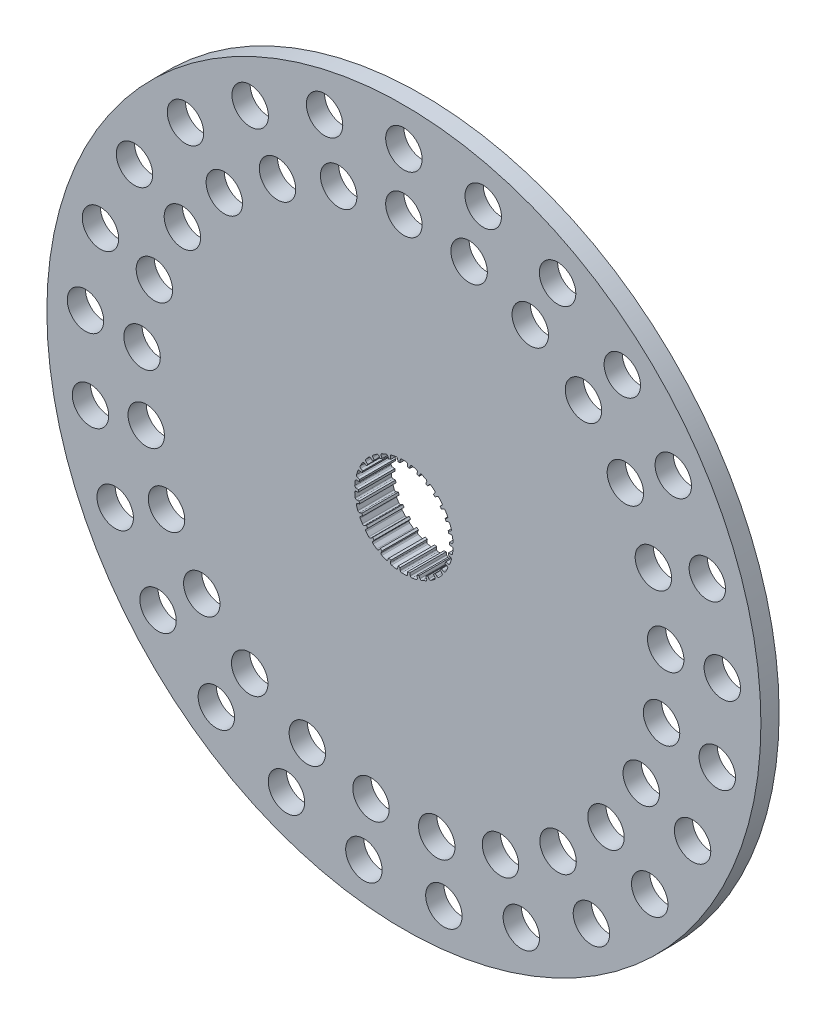
SolidWorks part; units mm, degrees
ref_plane "Front Plane" through (0, 0, 0) normal (0, 0, 1) x (1, 0, 0)
ref_plane "Top Plane" through (0, 0, 0) normal (0, 1, 0) x (1, 0, 0)
ref_plane "Right Plane" through (0, 0, 0) normal (1, 0, 0) x (0, 0, -1)
sketch "Sketch1" plane through (0, 0, 0) normal (0, 0, 1) x (1, 0, 0)
  circle A0 centre (0, 0) radius 98
  dimension "D1" = 196
extrude "Boss-Extrude1" add sketch "Sketch1" along normal blind 5
sketch "Sketch2" plane through (0, 0, 5) normal (0, 0, 1) x (1, 0, 0)
  line L0 (0, 0) -> (0, 103.0672) construction
  circle A0 centre (0, 87.5748) radius 5
  circle A1 centre (21.779, 84.8235) radius 5
  circle A2 centre (42.1895, 76.7424) radius 5
  circle A3 centre (59.9491, 63.8393) radius 5
  circle A4 centre (73.9419, 46.9249) radius 5
  circle A5 centre (83.2886, 27.0621) radius 5
  circle A6 centre (87.402, 5.4989) radius 5
  circle A7 centre (86.0237, -16.4099) radius 5
  circle A8 centre (79.2401, -37.2876) radius 5
  circle A9 centre (67.4776, -55.8223) radius 5
  circle A10 centre (51.4752, -70.8495) radius 5
  circle A11 centre (32.2384, -81.425) radius 5
  circle A12 centre (10.976, -86.8843) radius 5
  circle A13 centre (-10.976, -86.8843) radius 5
  circle A14 centre (-32.2384, -81.425) radius 5
  circle A15 centre (-51.4752, -70.8495) radius 5
  circle A16 centre (-67.4776, -55.8223) radius 5
  circle A17 centre (-79.2401, -37.2876) radius 5
  circle A18 centre (-86.0237, -16.4099) radius 5
  circle A19 centre (-87.402, 5.4989) radius 5
  circle A20 centre (-83.2886, 27.0621) radius 5
  circle A21 centre (-73.9419, 46.9249) radius 5
  circle A22 centre (-59.9491, 63.8393) radius 5
  circle A23 centre (-42.1895, 76.7424) radius 5
  circle A24 centre (-21.779, 84.8235) radius 5
  circle A25 centre (0, 72) radius 5
  circle A26 centre (17.9057, 69.738) radius 5
  circle A27 centre (34.6863, 63.0941) radius 5
  circle A28 centre (49.2874, 52.4857) radius 5
  circle A29 centre (60.7916, 38.5795) radius 5
  circle A30 centre (68.4761, 22.2492) radius 5
  circle A31 centre (71.8579, 4.5209) radius 5
  circle A32 centre (70.7247, -13.4915) radius 5
  circle A33 centre (65.1475, -30.6561) radius 5
  circle A34 centre (55.477, -45.8945) radius 5
  circle A35 centre (42.3205, -58.2492) radius 5
  circle A36 centre (26.505, -66.9439) radius 5
  circle A37 centre (9.024, -71.4323) radius 5
  circle A38 centre (-9.024, -71.4323) radius 5
  circle A39 centre (-26.505, -66.9439) radius 5
  circle A40 centre (-42.3205, -58.2492) radius 5
  circle A41 centre (-55.477, -45.8945) radius 5
  circle A42 centre (-65.1475, -30.6561) radius 5
  circle A43 centre (-70.7247, -13.4915) radius 5
  circle A44 centre (-71.8579, 4.5209) radius 5
  circle A45 centre (-68.4761, 22.2492) radius 5
  circle A46 centre (-60.7916, 38.5795) radius 5
  circle A47 centre (-49.2874, 52.4857) radius 5
  circle A48 centre (-34.6863, 63.0941) radius 5
  circle A49 centre (-17.9057, 69.738) radius 5
  point P51 (0, 0)
  point P107 (0, 0)
  dimension "D1" = 25
  dimension "D2" = 72
  dimension "D3" = 25
extrude "Cut-Extrude1" cut sketch "Sketch2" against normal blind 5
sketch "Sketch3" plane through (0, 0, 0) normal (0, 0, -1) x (-1, 0, 0)
  circle A1 centre (0, 0) radius 60.1971
ref_plane "Plane1" through (0, 0, -5) normal (0, 0, -1) x (-1, 0, 0)
sketch "Sketch4" plane through (0, 0, -5) normal (0, 0, -1) x (-1, 0, 0)
  circle A0 centre (0, 0) radius 40.1971
  circle A1 centre (0, 0) radius 60.1971 construction
  dimension "D1" = 20
loft "Loft1" add profiles "Sketch4", "Sketch3"
sketch "Sketch5" plane through (0, 0, -5) normal (0, 0, -1) x (-1, 0, 0)
  circle A0 centre (0, 0) radius 12.5
  dimension "D1" = 25
extrude "Cut-Extrude2" cut sketch "Sketch5" against normal through all
sketch "Sketch7" plane through (0, 0, -5) normal (0, 0, -1) x (-1, 0, 0)
  line L0 (0, 0) -> (0, 33.8861) construction
  line L2 (-0.6, 13.5) -> (0.6, 13.5)
  line L3 (-1, 13.1) -> (-1, 11.5)
  line L4 (-1, 11.5) -> (1, 11.5)
  line L5 (1, 13.1) -> (1, 11.5)
  line L6 (-1, 13.5) -> (1, 11.5) construction
  line L7 (-1, 11.5) -> (1, 13.5) construction
  circle A0 centre (0, 0) radius 12.5 construction
  arc A1 (1, 13.1) -> (0.6, 13.5) centre (0.6, 13.1) ccw
  arc A2 (-1, 13.1) -> (-0.6, 13.5) centre (-0.6, 13.1) cw
  point P3 (0, 12.5)
  dimension "D3" = 0.4
  dimension "D1" = 2
  dimension "D2" = 2
extrude "Cut-Extrude3" cut sketch "Sketch7" against normal through all
pattern_circular "CirPattern1" count 30 over 360 about axis through (0, 0, 0) along (0, 0, 1) of "Cut-Extrude3"
